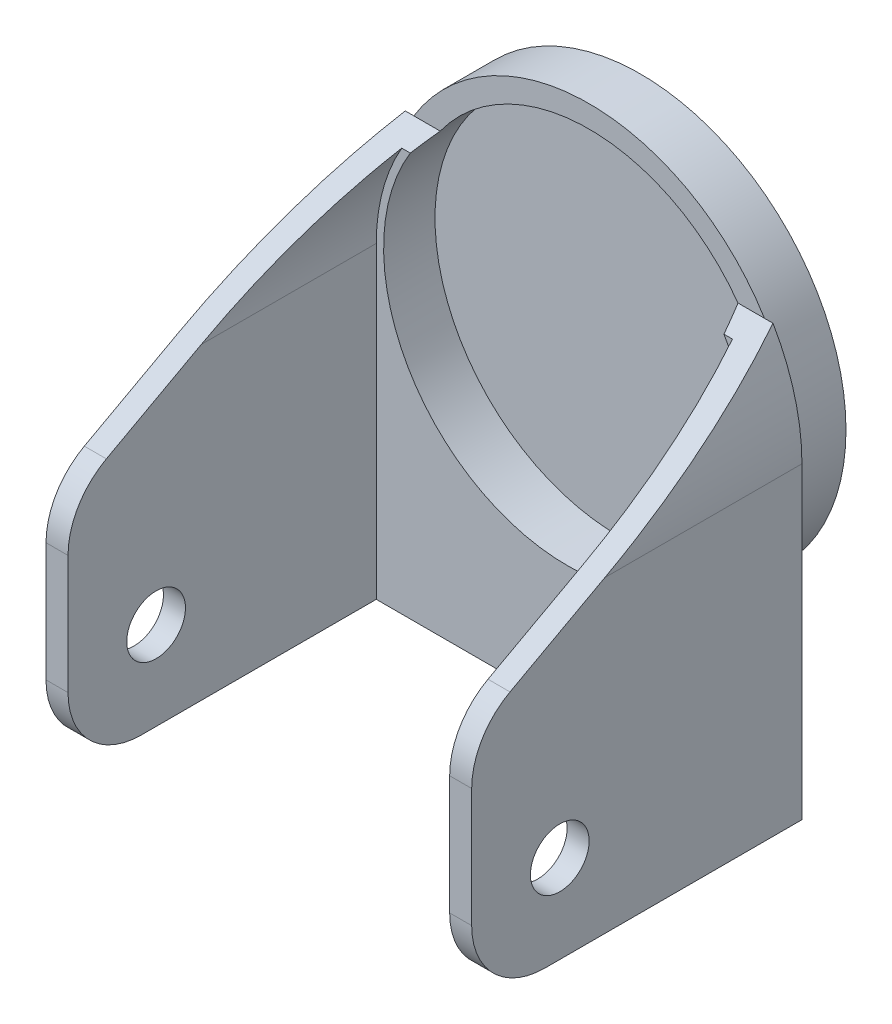
SolidWorks part; units mm, degrees
ref_plane "前视基准面" through (0, 0, 0) normal (0, 0, 1) x (1, 0, 0)
ref_plane "上视基准面" through (0, 0, 0) normal (0, 1, 0) x (1, 0, 0)
ref_plane "右视基准面" through (0, 0, 0) normal (1, 0, 0) x (0, 0, -1)
sketch "草图1" plane through (0, 0, 0) normal (0, 0, 1) x (1, 0, 0)
  circle A0 centre (0, 0) radius 12.5
  dimension "D1" = 25
extrude "凸台-拉伸1" add sketch "草图1" along normal blind 3
sketch "草图2" plane through (0, 0, 3) normal (0, 0, 1) x (1, 0, 0)
  circle A0 centre (0, 0) radius 28
  dimension "D1" = 56
extrude "凸台-拉伸2" add sketch "草图2" along normal blind 10
sketch "草图3" plane through (0, 0, 13) normal (0, 0, 1) x (1, 0, 0)
  circle A2 centre (0, 0) radius 25
  circle A3 centre (0, 0) radius 25
  dimension "D1" = 3
extrude "切除-拉伸1" cut sketch "草图3" against normal blind 7
sketch "草图6" plane through (0, 0, 13) normal (0, 0, 1) x (1, 0, 0)
  circle A0 centre (0, 0) radius 25 construction
  circle A1 centre (0, 0) radius 25
  circle A2 centre (0, 0) radius 29
  dimension "D1" = 58
extrude "凸台-拉伸4" add sketch "草图6" against normal blind 3
sketch "草图4" plane through (0, 0, 13) normal (0, 0, 1) x (1, 0, 0)
  line L0 (-29, 0) -> (-29, -42)
  line L1 (-29, -42) -> (29, -42)
  line L2 (29, 0) -> (29, -42)
  circle A0 centre (0, 0) radius 28 construction
  circle A1 centre (0, 0) radius 29 construction
  dimension "D1" = 71
extrude "凸台-拉伸3" add sketch "草图4" against normal blind 3
sketch "草图7" plane through (0, 0, 13) normal (0, 0, 1) x (1, 0, 0)
  line L0 (-26, 0) -> (-26, -42)
  line L1 (-26, 0) -> (-26, -39) construction
  line L2 (26, -42) -> (26, 0)
  line L3 (-29, 0) -> (-29, -42)
  line L4 (-29, -42) -> (29, -42)
  line L5 (29, -42) -> (29, 0)
  line L6 (-29, 0) -> (-29, -42)
  line L7 (-29, -42) -> (29, -42)
  line L8 (29, -42) -> (29, 0)
  line L9 (-26, -39) -> (26, -39) construction
  line L10 (26, -39) -> (26, 0) construction
  arc A0 (26, 0) -> (-26, 0) centre (0, 0) ccw
  arc A1 (29, 0) -> (-29, 0) centre (0, 0) ccw
  arc A2 (29, 0) -> (-29, 0) centre (0, 0) ccw
  arc M6 (29, 0) -> (-29, 0) centre (0, 0) ccw
  line M7 (-29, 0) -> (-29, -42)
  line M8 (-29, -42) -> (29, -42)
  line M9 (29, -42) -> (29, 0)
  dimension "D1" = 0
  dimension "D2" = 3
extrude "凸台-拉伸5" add sketch "草图7" along normal blind 42 contours A0 L2 L0 M8 M9 M6 M7
sketch "草图8" plane through (29, 0, 0) normal (1, 0, 0) x (0, 0, -1)
  line L0 (-55, -9.8725) -> (-10, 14.6097)
  line L1 (-55, -42) -> (-55, 0) construction
  line L2 (-10, -28) -> (-10, 28) construction
  line L3 (-10, 14.6097) -> (-10, 29)
  line L4 (-10, 29) -> (-55, 29)
  line L5 (-55, 29) -> (-55, -9.8725)
extrude "切除-拉伸2" cut sketch "草图8" against normal through all
fillet "圆角1" radius 10 4 edges at (27.5, -9.8725, 55) (27.5, -42, 55) (-27.5, -9.8725, 55) (-27.5, -42, 55)
sketch "草图9" plane through (29, 0, 0) normal (1, 0, 0) x (0, 0, -1)
  line L0 (0, -12.5) -> (0, 12.5) construction
  circle A0 centre (-43, -30) radius 4
  dimension "D1" = 43
  dimension "D3" = 8
  dimension "D2" = 30
extrude "切除-拉伸4" cut sketch "草图9" against normal through all
